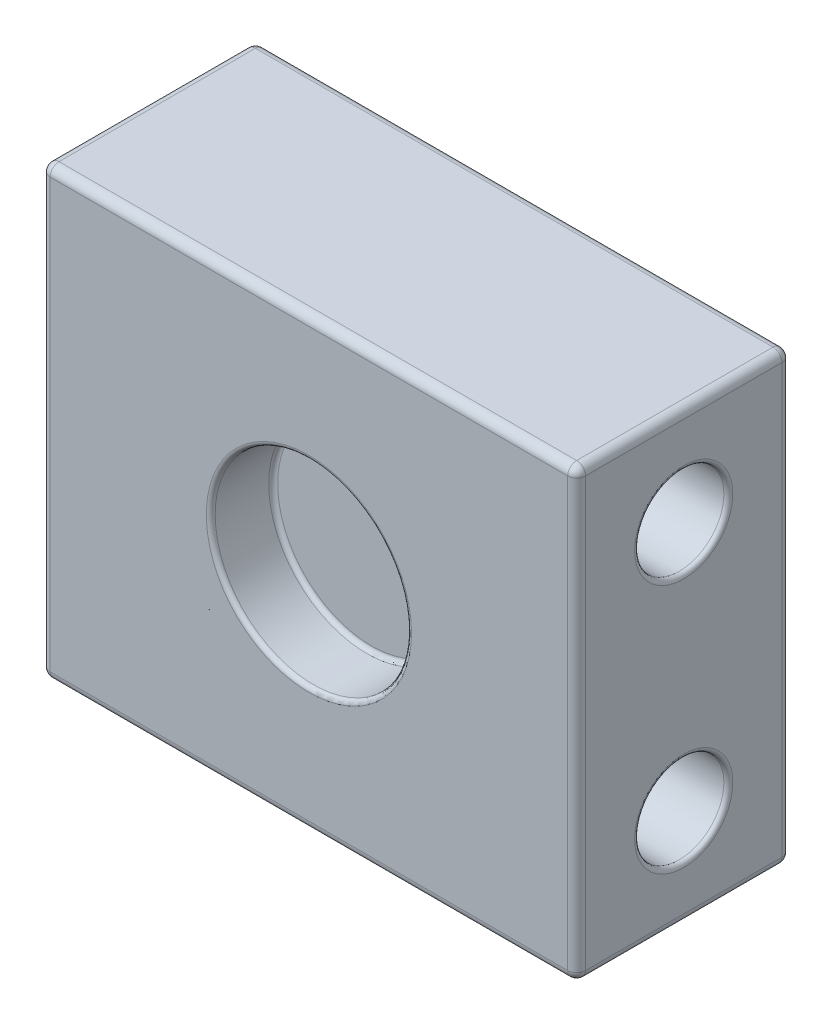
from build123d import *

# Parameters (mm, degrees)
SKETCH1_W           = 60
SKETCH1_H           = 50
BOSS_EXTRUDE1_DEPTH = 12
SKETCH2_R           = 11
CUT_EXTRUDE1_DEPTH  = 7
SKETCH3_R           = 5
CUT_EXTRUDE2_DEPTH  = 67.098411479
FILLET1_R           = 1
FILLET2_R           = 0.5


with BuildPart() as part:
    # Sketch1 → Boss-Extrude1 (new, symmetric)
    with BuildSketch(Plane.XY):
        Rectangle(SKETCH1_W, SKETCH1_H)
    extrude(amount=BOSS_EXTRUDE1_DEPTH, both=True)

    # Sketch2 → Cut-Extrude1 (cut)
    with BuildSketch(Plane.XY.offset(12)):
        Circle(SKETCH2_R)
    extrude(amount=-CUT_EXTRUDE1_DEPTH, mode=Mode.SUBTRACT)

    # Sketch3 → Cut-Extrude2 (cut, through all)
    with BuildSketch(Plane(origin=(30, 0, 0), x_dir=(0, 0, -1), z_dir=(1, 0, 0))):
        with Locations((0, 14)):
            Circle(SKETCH3_R)
        with Locations((0, -14)):
            Circle(SKETCH3_R)
    extrude(amount=-CUT_EXTRUDE2_DEPTH, mode=Mode.SUBTRACT)

    # Fillet1
    fillet1_edges = [part.edges().sort_by_distance(p)[0] for p in [
        (30, 0, 12),
        (0, 25, 12),
        (-30, 0, 12),
        (0, 25, -12),
        (30, 0, -12),
        (0, -25, -12),
        (-30, 0, -12),
        (0, -25, 12),
        (-30, 25, 0),
        (30, 25, 0),
        (30, -25, 0),
        (-30, -25, 0),
    ]]
    fillet(fillet1_edges, radius=FILLET1_R)

    # Fillet2
    fillet2_edges = [part.edges().sort_by_distance(p)[0] for p in [
        (-11, 0, 5),
        (-11, 0, 12),
        (-30, 14, 5),
        (30, 14, 5),
        (-30, -14, 5),
        (30, -14, 5),
    ]]
    fillet(fillet2_edges, radius=FILLET2_R)


solid = part.part
